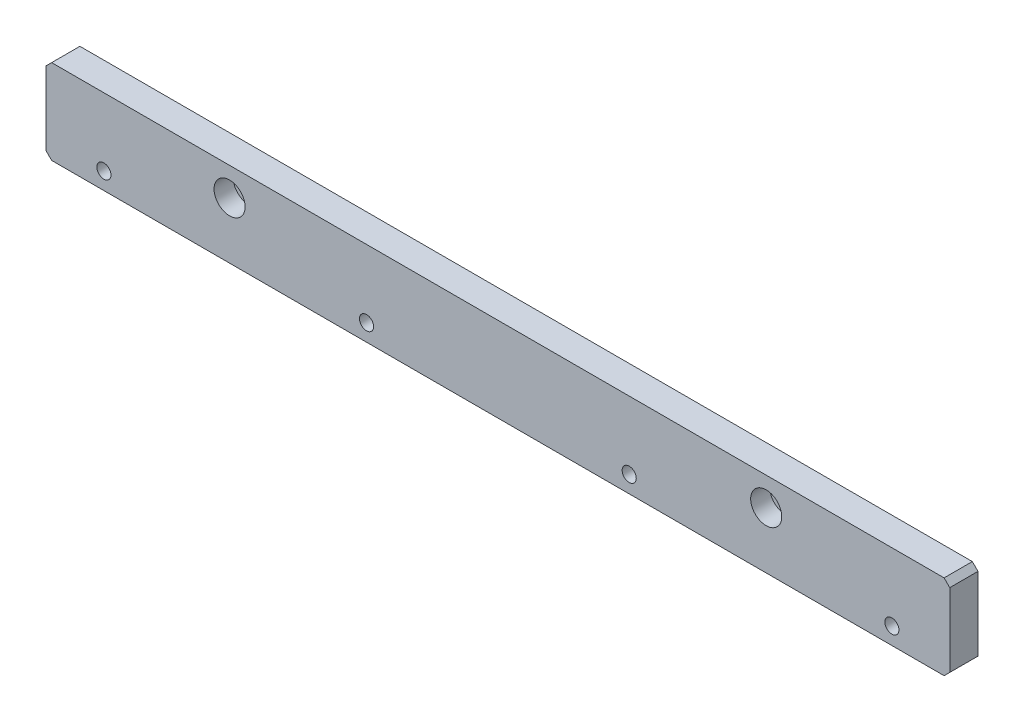
SolidWorks part; units mm, degrees
material "Q235-A"
ref_plane "Front Plane" through (0, 0, 0) normal (0, 0, 1) x (1, 0, 0)
ref_plane "Top Plane" through (0, 0, 0) normal (0, 1, 0) x (1, 0, 0)
ref_plane "Right Plane" through (0, 0, 0) normal (1, 0, 0) x (0, 0, -1)
sketch "Sketch1" plane through (0, 0, 0) normal (0, 0, 1) x (1, 0, 0)
  line L1 (-160, -15) -> (160, -15)
  line L2 (-160, -15) -> (-160, 15)
  line L3 (-160, 15) -> (160, 15)
  line L4 (160, -15) -> (160, 15)
  line L5 (-160, -15) -> (160, 15) construction
  line L6 (-160, 15) -> (160, -15) construction
  point P0 (0, 0)
  dimension "D1" = 320
  dimension "D2" = 30
extrude "Boss-Extrude1" add sketch "Sketch1" along normal blind 10
chamfer "Chamfer1" distance 2 angle 45 4 edges at (160, -15, 5) (160, 15, 5) (-160, -15, 5) (-160, 15, 5)
sketch "Sketch2" plane through (0, 0, 10) normal (0, 0, 1) x (1, 0, 0)
  line L0 (-95, 5) -> (95, 5)
  line L1 (-160, 13) -> (-160, -13) construction
  line L2 (-158, -15) -> (158, -15) construction
  point P6 (-139.5, -9)
  point P9 (-46.5, -9)
  point P10 (46.5, -9)
  point P11 (139.5, -9)
  dimension "D1" = 190
  dimension "D2" = 65
  dimension "D3" = 20
  dimension "D4" = 6
  dimension "D5" = 20.5
  dimension "D6" = 4
hole_wizard "M6 Tapped Hole1" positions "Sketch3" profile "Sketch4" tap size "M6" standard "GB" end condition through all
sketch "Sketch3" plane through (0, 0, 10) normal (0, 0, 1) x (1, 0, 0)
  point P0 (-139.5, -9)
  point P3 (-46.5, -9)
  point P6 (46.5, -9)
  point P9 (139.5, -9)
sketch "Sketch4" plane through (-139.5, -9, 10) normal (1, 0, 0) x (0, -1, 0)
  line L0 (0, 0) -> (0, 10)
  line L1 (0, 10) -> (2.5, 10)
  line L2 (2.5, 10) -> (2.5, 0)
  line L5 (2.5, 0) -> (0, 0)
  line L11 (0, -6.35) -> (0, 107.95) construction
  dimension "通孔螺纹孔钻头直径" = 5
  dimension "通孔螺纹孔钻头深度" = 10
cosmetic thread "Cosmetic Thread1"
cosmetic thread "Cosmetic Thread2"
cosmetic thread "Cosmetic Thread3"
cosmetic thread "Cosmetic Thread4"
hole_wizard "Hole1" positions "Sketch5" profile "Sketch6" legacy end condition through all
sketch "Sketch5" plane through (0, 0, 10) normal (0, 0, 1) x (1, 0, 0)
  point P0 (-95, 5)
  point P3 (95, 5)
sketch "Sketch6" plane through (-95, 5, 10) normal (1, 0, 0) x (0, -1, 0)
  line L0 (0, 0) -> (0, 10)
  line L1 (0, 10) -> (3.3, 10)
  line L2 (3.3, 10) -> (3.3, 6.8)
  line L3 (3.3, 6.8) -> (5.5, 6.8)
  line L4 (5.5, 6.8) -> (5.5, 0)
  line L5 (5.5, 0) -> (0, 0)
  line L6 (0, 110) -> (0, -10) construction
  dimension "直径" = 6.6
  dimension "深度" = 10
  dimension "柱坑直径" = 11
  dimension "柱坑深度" = 6.8
